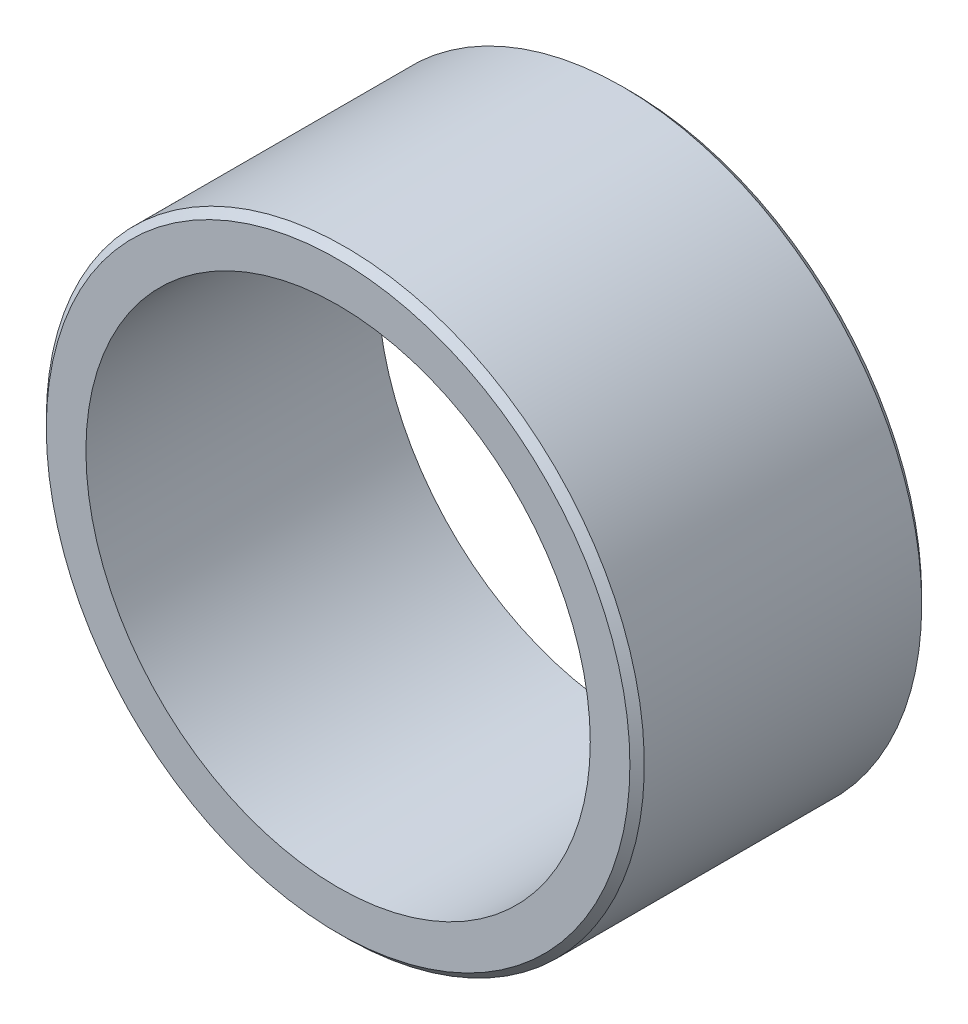
SolidWorks part; units mm, degrees
material "普通碳钢"
ref_plane "Front Plane" through (0, 0, 0) normal (0, 0, 1) x (1, 0, 0)
ref_plane "Top Plane" through (0, 0, 0) normal (0, 1, 0) x (1, 0, 0)
ref_plane "Right Plane" through (0, 0, 0) normal (1, 0, 0) x (0, 0, -1)
sketch "Sketch1" plane through (0, 0, 0) normal (0, 0, 1) x (1, 0, 0)
  circle A0 centre (0, 0) radius 41.5
  circle A1 centre (0, 0) radius 35
  dimension "D1" = 83
  dimension "D2" = 70
extrude "Extrude1" add sketch "Sketch1" along normal blind 40.5
chamfer "Chamfer1" distance 1 angle 45 2 edges at (41.5, 0, 0) (41.5, 0, 40.5)
